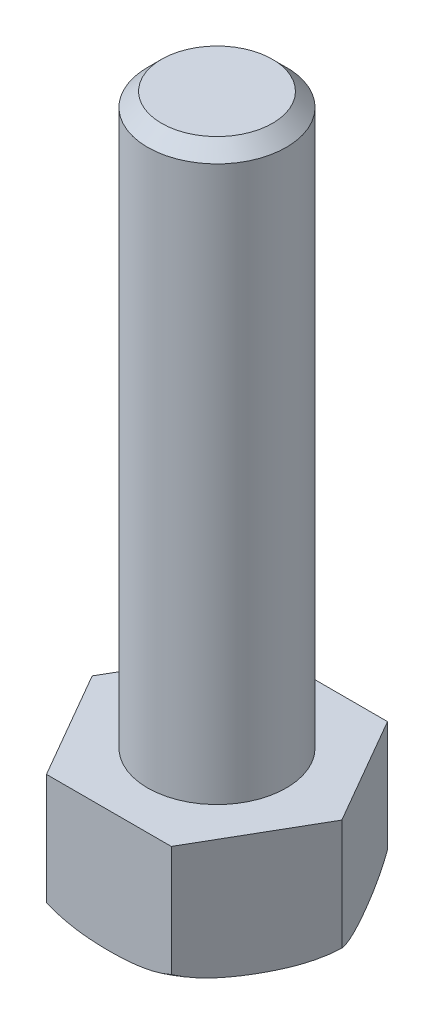
from build123d import *

# Parameters (mm, degrees)
SKETCH2_OUTSIDE_W  = 31.222
SKETCH2_OUTSIDE_H  = 31.222
CUT_EXTRUDE2_DEPTH = 10
SCALE_1_SCALE      = 1.875


with BuildPart() as part:
    # Sketch1 → Revolve1 (revolve)
    with BuildSketch(Plane.XY, mode=Mode.PRIVATE) as revolve1_sk:
        Polygon((0, 0), (9, 0), (9, 9), (5, 9), (5, 49), (4, 50), (0, 50), align=None)
    revolve(revolve1_sk.sketch.rotate(Axis((0, 50, 0), (0, -1, 0)), 90), axis=Axis((0, 50, 0), (0, -1, 0)))

    # Sketch2 outside → Cut-Extrude2 (cut)
    with BuildSketch(Plane.XZ):
        Rectangle(SKETCH2_OUTSIDE_W, SKETCH2_OUTSIDE_H)
        Polygon((9, 0), (4.5, 7.794228634), (-4.5, 7.794228634), (-9, 0), (-4.5, -7.794228634), (4.5, -7.794228634), align=None, mode=Mode.SUBTRACT)
    extrude(amount=-CUT_EXTRUDE2_DEPTH, mode=Mode.SUBTRACT)

    # Sketch5 → Cut-Revolve2 (revolve, cut)
    with BuildSketch(Plane.XY, mode=Mode.PRIVATE) as cut_revolve2_sk:
        with BuildLine():
            Line((-9, 0), (-9, 1))
            ThreePointArc((-9, 1), (-8.071297978, 0.357404043), (-7, 0))
            Line((-7, 0), (-9, 0))
        make_face()
    revolve(cut_revolve2_sk.sketch.rotate(Axis((0, 0, 0), (0, 1, 0)), 270), axis=Axis((0, 0, 0), (0, 1, 0)), mode=Mode.SUBTRACT)


with BuildPart() as part_1:
    # Scale 1: scaled about (-2.65e-07, 20.203740947, 0)
    add(part.part.scale(SCALE_1_SCALE).moved(Location((2.32e-07, -17.678273329, 0))))


solid = part_1.part
